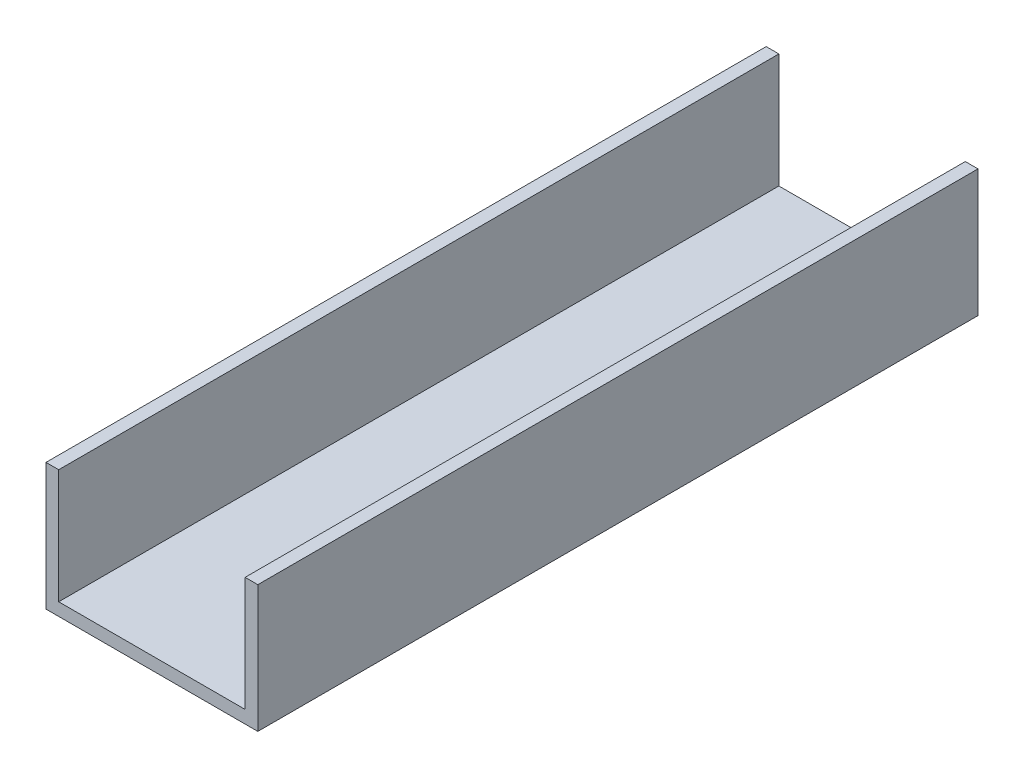
SolidWorks part; units mm, degrees
ref_plane "前视基准面" through (0, 0, 0) normal (0, 0, 1) x (1, 0, 0)
ref_plane "上视基准面" through (0, 0, 0) normal (0, 1, 0) x (1, 0, 0)
ref_plane "右视基准面" through (0, 0, 0) normal (1, 0, 0) x (0, 0, -1)
sketch "草图1" plane through (0, 0, 0) normal (0, 0, 1) x (1, 0, 0)
  line L0 (0, 0) -> (0, 30)
  line L1 (0, 0) -> (50, 0)
  line L2 (50, 0) -> (50, 30)
  line L3 (47, 3) -> (47, 30)
  line L4 (3, 3) -> (47, 3)
  line L5 (3, 3) -> (3, 30)
  line L6 (0, 30) -> (3, 30)
  line L7 (47, 30) -> (50, 30)
  dimension "D1" = 3
extrude "凸台-拉伸1" add sketch "草图1" along normal blind 340
sketch "草图2" plane through (0, 0, 340) normal (0, 0, 1) x (1, 0, 0)
  line L16 (0, 0) -> (50, 0)
  line L17 (50, 0) -> (50, 30)
  line L18 (50, 30) -> (47, 30)
  line L19 (47, 30) -> (47, 3)
  line L20 (47, 3) -> (3, 3)
  line L21 (3, 3) -> (3, 30)
  line L22 (3, 30) -> (0, 30)
  line L23 (0, 30) -> (0, 0)
  line L24 (0, 0) -> (50, 0)
  line L25 (50, 0) -> (50, 30)
  line L26 (50, 30) -> (47, 30)
  line L27 (47, 30) -> (47, 3)
  line L28 (47, 3) -> (3, 3)
  line L29 (3, 3) -> (3, 30)
  line L30 (3, 30) -> (0, 30)
  line L31 (0, 30) -> (0, 0)
  dimension "D1" = 0
extrude "切除-拉伸1" cut sketch "草图2" against normal blind 170
